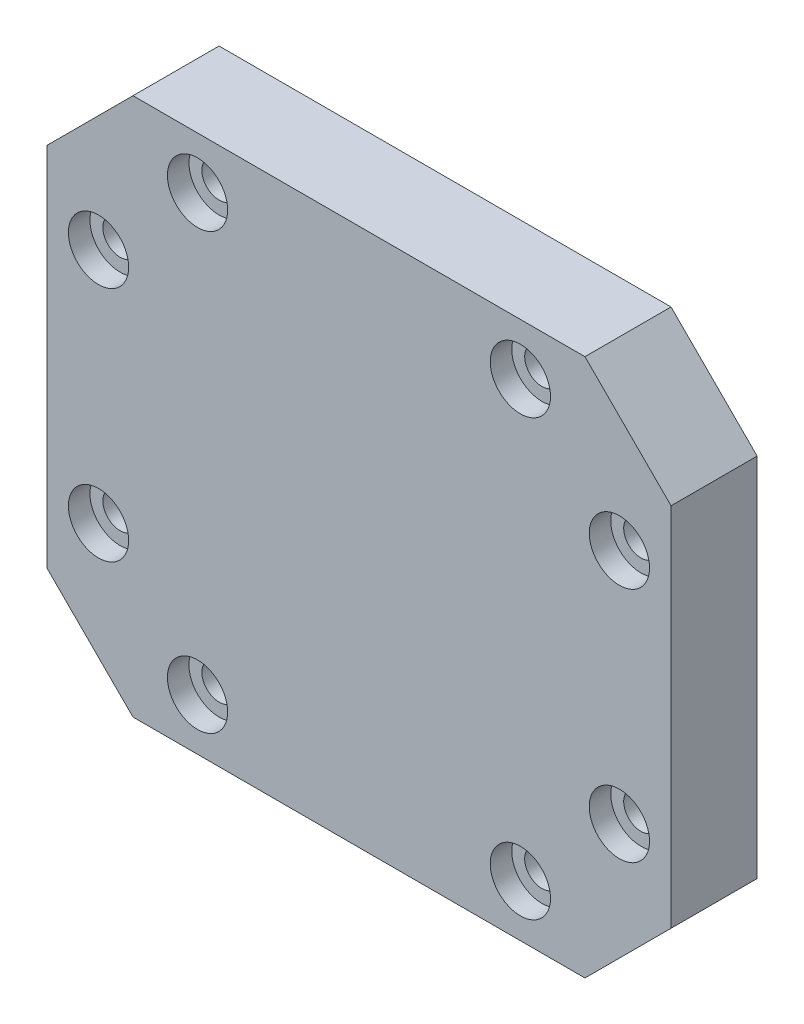
from build123d import *

# Parameters (mm, degrees)
SKETCH_1_W          = 145
SKETCH_1_H          = 125
EXTRUDE_1_DEPTH     = 20
CHAMFER_1_SIZE      = 20
SKETCH_2_R          = 7
CUT_EXTRUDE_1_DEPTH = 5
CUT_EXTRUDE_2_REACH = 98.889
SKETCH_3_R          = 4
SKETCH_4_W          = 38
SKETCH_4_H          = 31
CUT_EXTRUDE_3_DEPTH = 1.5
SKETCH_5_R          = 2.5
CUT_EXTRUDE_4_DEPTH = 1.5


with BuildPart() as part:
    # 草图1 → 凸台-拉伸1 (new body)
    with BuildSketch(Plane.XY):
        Rectangle(SKETCH_1_W, SKETCH_1_H)
    extrude(amount=EXTRUDE_1_DEPTH)

    # 倒角1
    chamfer_1_edges = [part.edges().sort_by_distance(p)[0] for p in [
        (72.5, -62.5, 10),
        (-72.5, -62.5, 10),
        (-72.5, 62.5, 10),
        (72.5, 62.5, 10),
    ]]
    chamfer(chamfer_1_edges, length=CHAMFER_1_SIZE)

    # 草图2 → 切除-拉伸1 (cut)
    with BuildSketch(Plane.XY.offset(20)):
        with Locations((-37.5, 50.5)):
            Circle(SKETCH_2_R)
        with Locations((37.5, 50.5)):
            Circle(SKETCH_2_R)
        with Locations((-60.5, 27.5)):
            Circle(SKETCH_2_R)
        with Locations((-60.5, -27.5)):
            Circle(SKETCH_2_R)
        with Locations((-37.5, -50.5)):
            Circle(SKETCH_2_R)
        with Locations((37.5, -50.5)):
            Circle(SKETCH_2_R)
        with Locations((60.5, 27.5)):
            Circle(SKETCH_2_R)
        with Locations((60.5, -27.5)):
            Circle(SKETCH_2_R)
    extrude(amount=-CUT_EXTRUDE_1_DEPTH, mode=Mode.SUBTRACT)

    # 草图3 → 切除-拉伸2 (cut, up to next)
    with BuildSketch(Plane.XY.offset(15), mode=Mode.PRIVATE) as cut_extrude_2_sk1:
        with Locations((-37.5, 50.5)):
            Circle(SKETCH_3_R)
    cut_extrude_2_tool1 = extrude(cut_extrude_2_sk1.sketch, amount=-CUT_EXTRUDE_2_REACH, mode=Mode.PRIVATE) & part.part
    # 草图3 → 切除-拉伸2 (cut, up to next)
    with BuildSketch(Plane.XY.offset(15), mode=Mode.PRIVATE) as cut_extrude_2_sk2:
        with Locations((-60.5, 27.5)):
            Circle(SKETCH_3_R)
    cut_extrude_2_tool2 = extrude(cut_extrude_2_sk2.sketch, amount=-CUT_EXTRUDE_2_REACH, mode=Mode.PRIVATE) & part.part
    # 草图3 → 切除-拉伸2 (cut, up to next)
    with BuildSketch(Plane.XY.offset(15), mode=Mode.PRIVATE) as cut_extrude_2_sk3:
        with Locations((-60.5, -27.5)):
            Circle(SKETCH_3_R)
    cut_extrude_2_tool3 = extrude(cut_extrude_2_sk3.sketch, amount=-CUT_EXTRUDE_2_REACH, mode=Mode.PRIVATE) & part.part
    # 草图3 → 切除-拉伸2 (cut, up to next)
    with BuildSketch(Plane.XY.offset(15), mode=Mode.PRIVATE) as cut_extrude_2_sk4:
        with Locations((-37.5, -50.5)):
            Circle(SKETCH_3_R)
    cut_extrude_2_tool4 = extrude(cut_extrude_2_sk4.sketch, amount=-CUT_EXTRUDE_2_REACH, mode=Mode.PRIVATE) & part.part
    # 草图3 → 切除-拉伸2 (cut, up to next)
    with BuildSketch(Plane.XY.offset(15), mode=Mode.PRIVATE) as cut_extrude_2_sk5:
        with Locations((37.5, 50.5)):
            Circle(SKETCH_3_R)
    cut_extrude_2_tool5 = extrude(cut_extrude_2_sk5.sketch, amount=-CUT_EXTRUDE_2_REACH, mode=Mode.PRIVATE) & part.part
    # 草图3 → 切除-拉伸2 (cut, up to next)
    with BuildSketch(Plane.XY.offset(15), mode=Mode.PRIVATE) as cut_extrude_2_sk6:
        with Locations((60.5, 27.5)):
            Circle(SKETCH_3_R)
    cut_extrude_2_tool6 = extrude(cut_extrude_2_sk6.sketch, amount=-CUT_EXTRUDE_2_REACH, mode=Mode.PRIVATE) & part.part
    # 草图3 → 切除-拉伸2 (cut, up to next)
    with BuildSketch(Plane.XY.offset(15), mode=Mode.PRIVATE) as cut_extrude_2_sk7:
        with Locations((60.5, -27.5)):
            Circle(SKETCH_3_R)
    cut_extrude_2_tool7 = extrude(cut_extrude_2_sk7.sketch, amount=-CUT_EXTRUDE_2_REACH, mode=Mode.PRIVATE) & part.part
    # 草图3 → 切除-拉伸2 (cut, up to next)
    with BuildSketch(Plane.XY.offset(15), mode=Mode.PRIVATE) as cut_extrude_2_sk8:
        with Locations((37.5, -50.5)):
            Circle(SKETCH_3_R)
    cut_extrude_2_tool8 = extrude(cut_extrude_2_sk8.sketch, amount=-CUT_EXTRUDE_2_REACH, mode=Mode.PRIVATE) & part.part
    add(cut_extrude_2_tool1.solids().sort_by_distance((-37.5, 50.5, 15))[0], mode=Mode.SUBTRACT)
    add(cut_extrude_2_tool2.solids().sort_by_distance((-60.5, 27.5, 15))[0], mode=Mode.SUBTRACT)
    add(cut_extrude_2_tool3.solids().sort_by_distance((-60.5, -27.5, 15))[0], mode=Mode.SUBTRACT)
    add(cut_extrude_2_tool4.solids().sort_by_distance((-37.5, -50.5, 15))[0], mode=Mode.SUBTRACT)
    add(cut_extrude_2_tool5.solids().sort_by_distance((37.5, 50.5, 15))[0], mode=Mode.SUBTRACT)
    add(cut_extrude_2_tool6.solids().sort_by_distance((60.5, 27.5, 15))[0], mode=Mode.SUBTRACT)
    add(cut_extrude_2_tool7.solids().sort_by_distance((60.5, -27.5, 15))[0], mode=Mode.SUBTRACT)
    add(cut_extrude_2_tool8.solids().sort_by_distance((37.5, -50.5, 15))[0], mode=Mode.SUBTRACT)

    # 草图4 → 切除-拉伸3 (cut)
    with BuildSketch(Plane(origin=(0, 0, 0), x_dir=(-1, 0, 0), z_dir=(0, 0, -1))):
        Rectangle(SKETCH_4_W, SKETCH_4_H)
    extrude(amount=-CUT_EXTRUDE_3_DEPTH, mode=Mode.SUBTRACT)

    # 草图5 → 切除-拉伸4 (cut)
    with BuildSketch(Plane(origin=(0, 0, 0), x_dir=(-1, 0, 0), z_dir=(0, 0, -1))):
        with Locations((19, -15.5)):
            Circle(SKETCH_5_R)
        with Locations((-19, -15.5)):
            Circle(SKETCH_5_R)
        with Locations((-19, 15.5)):
            Circle(SKETCH_5_R)
        with Locations((19, 15.5)):
            Circle(SKETCH_5_R)
    extrude(amount=-CUT_EXTRUDE_4_DEPTH, mode=Mode.SUBTRACT)


solid = part.part
